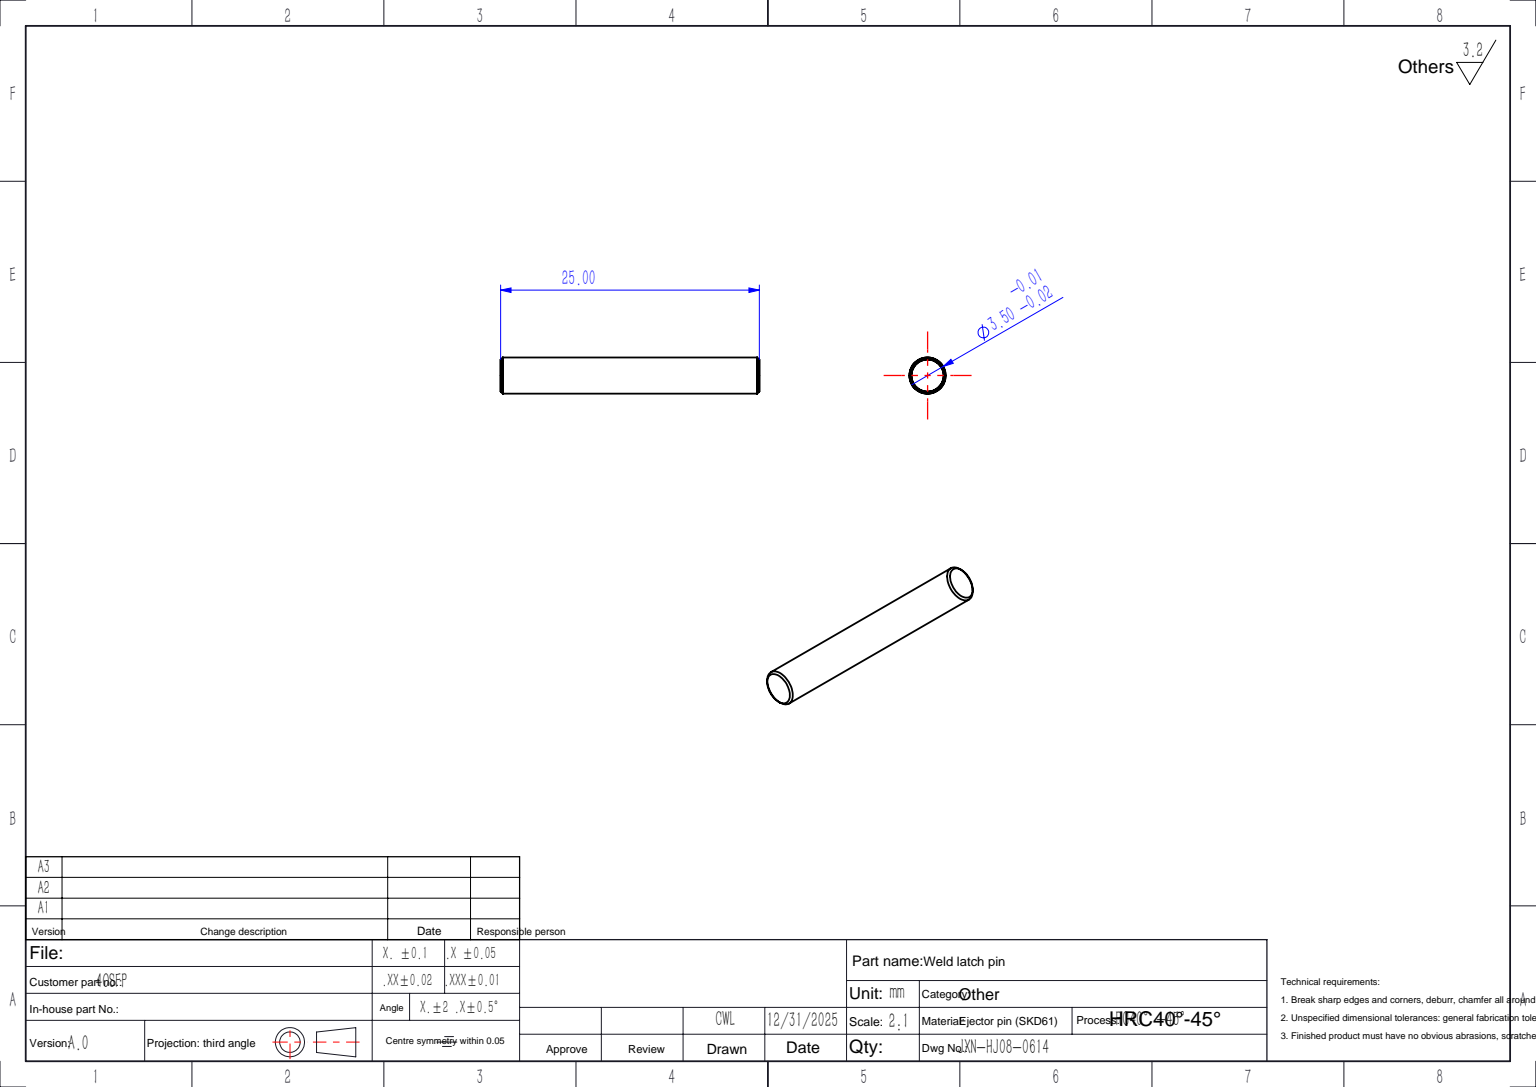
from build123d import *

# Parameters (mm, degrees)
SKETCH_1_R      = 1.75
EXTRUDE_1_DEPTH = 25
CHAMFER_1_SIZE  = 0.2


with BuildPart() as part:
    # 草图1 → 凸台-拉伸1 (new body)
    with BuildSketch(Plane(origin=(0, 0, 0), x_dir=(1, 0, 0), z_dir=(0, 1, 0))):
        with Locations(Location((0, 0, 0), (0, 0, 270))):
            Circle(SKETCH_1_R)
    extrude(amount=EXTRUDE_1_DEPTH)

    # 倒角1
    chamfer_1_edges = [part.edges().sort_by_distance(p)[0] for p in [
        (0, 0, -1.75),
        (0, 25, -1.75),
    ]]
    chamfer(chamfer_1_edges, length=CHAMFER_1_SIZE)


solid = part.part
